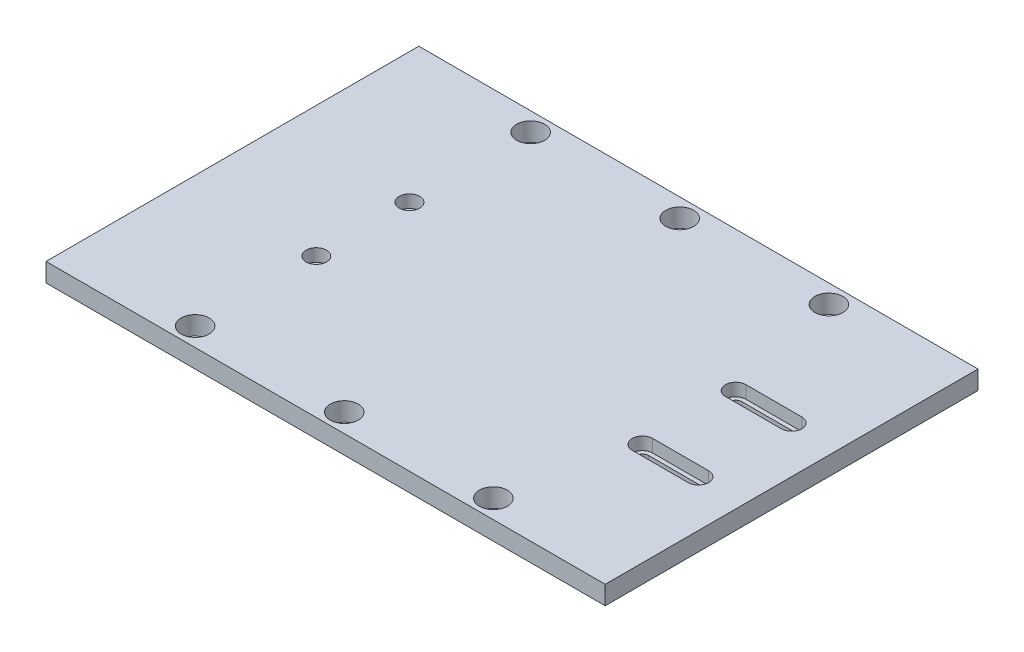
from build123d import *

# Parameters (mm, degrees)
SKETCH1_W                                           = 300
SKETCH1_H                                           = 200
BOSS_EXTRUDE1_DEPTH                                 = 5
SKETCH2_R                                           = 7.5
CUT_EXTRUDE1_DEPTH                                  = 10
LPATTERN1_COUNT                                     = 2
LPATTERN1_PITCH                                     = 180
LPATTERN1_COUNT_DIR2                                = 3
LPATTERN1_PITCH_DIR2                                = 80
HOLE_SIZE_BASED_ON_SOCKET_HEAD_CAP_SCRE_D           = 6.6
HOLE_SIZE_BASED_ON_SOCKET_HEAD_CAP_SCRE_CBORE_D     = 11
HOLE_SIZE_BASED_ON_SOCKET_HEAD_CAP_SCRE_CBORE_DEPTH = 6.8
CUT_EXTRUDE2_DEPTH                                  = 10
CUT_EXTRUDE3_DEPTH                                  = 6.8


with BuildPart() as part:
    # Sketch1 → Boss-Extrude1 (new, symmetric)
    with BuildSketch(Plane(origin=(0, 0, 0), x_dir=(1, 0, 0), z_dir=(0, 1, 0))):
        Rectangle(SKETCH1_W, SKETCH1_H)
    extrude(amount=BOSS_EXTRUDE1_DEPTH, both=True)

    # Sketch2 → Cut-Extrude1 (cut)
    with BuildSketch(Plane(origin=(0, 5, 0), x_dir=(1, 0, 0), z_dir=(0, 1, 0))):
        with Locations(Location((80, 90, 0), (0, 0, 270))):
            Circle(SKETCH2_R)
    cut_extrude1 = extrude(amount=-CUT_EXTRUDE1_DEPTH, mode=Mode.SUBTRACT)

    # LPattern1: Cut-Extrude1 2 × 3
    with Locations(*[(-j * LPATTERN1_PITCH_DIR2, 0, i * LPATTERN1_PITCH) for i in range(LPATTERN1_COUNT) for j in range(LPATTERN1_COUNT_DIR2) if (i, j) != (0, 0)]):
        add(cut_extrude1, mode=Mode.SUBTRACT)

    # Hole Size (based on socket head cap screw type)1 (through all)
    with Locations(Plane(origin=(0, 5, 0), x_dir=(1, 0, 0), z_dir=(0, 1, 0))):
        with Locations((-80, 25), (-80, -25)):
            CounterBoreHole(HOLE_SIZE_BASED_ON_SOCKET_HEAD_CAP_SCRE_D / 2, HOLE_SIZE_BASED_ON_SOCKET_HEAD_CAP_SCRE_CBORE_D / 2, HOLE_SIZE_BASED_ON_SOCKET_HEAD_CAP_SCRE_CBORE_DEPTH)

    # Sketch6 → Cut-Extrude2 (cut)
    with BuildSketch(Plane(origin=(0, 5, 0), x_dir=(1, 0, 0), z_dir=(0, 1, 0))):
        with BuildLine():
            Line((125, 21.7), (95, 21.7))
            ThreePointArc((95, 21.7), (91.7, 25), (95, 28.3))
            Line((95, 28.3), (125, 28.3))
            ThreePointArc((125, 28.3), (128.3, 25), (125, 21.7))
        make_face()
        with BuildLine():
            Line((125, -28.3), (95, -28.3))
            ThreePointArc((95, -28.3), (91.7, -25), (95, -21.7))
            Line((95, -21.7), (125, -21.7))
            ThreePointArc((125, -21.7), (128.3, -25), (125, -28.3))
        make_face()
    extrude(amount=-CUT_EXTRUDE2_DEPTH, mode=Mode.SUBTRACT)

    # Sketch7 → Cut-Extrude3 (cut)
    with BuildSketch(Plane(origin=(0, 5, 0), x_dir=(1, 0, 0), z_dir=(0, 1, 0))):
        with BuildLine():
            Line((125, 19.5), (95, 19.5))
            ThreePointArc((95, 19.5), (89.5, 25), (95, 30.5))
            Line((95, 30.5), (125, 30.5))
            ThreePointArc((125, 30.5), (130.5, 25), (125, 19.5))
        make_face()
        with BuildLine():
            Line((125, -30.5), (95, -30.5))
            ThreePointArc((95, -30.5), (89.5, -25), (95, -19.5))
            Line((95, -19.5), (125, -19.5))
            ThreePointArc((125, -19.5), (130.5, -25), (125, -30.5))
        make_face()
    extrude(amount=-CUT_EXTRUDE3_DEPTH, mode=Mode.SUBTRACT)


solid = part.part
